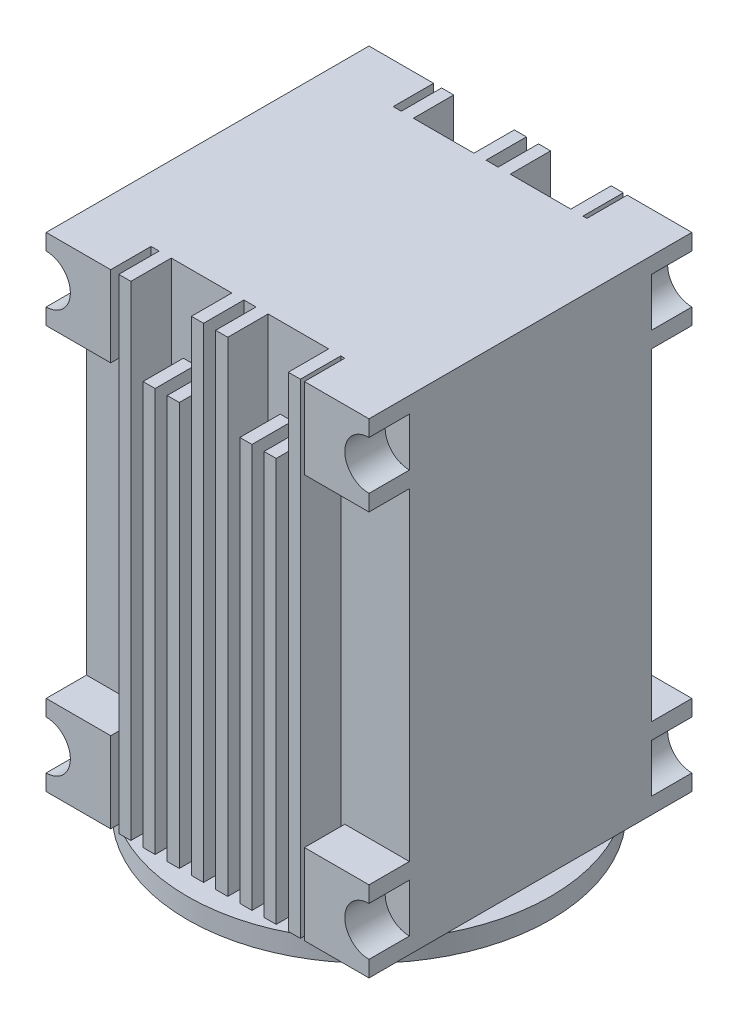
from build123d import *

# Parameters (mm, degrees)
SKETCH1_W           = 40
SKETCH1_H           = 40
BOSS_EXTRUDE1_DEPTH = 30
CUT_EXTRUDE1_DEPTH  = 5
SKETCH3_W           = 1.5
SKETCH3_H           = 5
BOSS_EXTRUDE2_DEPTH = 60
SKETCH4_W           = 4.5
SKETCH4_H           = 10
CUT_EXTRUDE2_DEPTH  = 5
SKETCH5_R           = 3
CUT_EXTRUDE3_DEPTH  = 5
SKETCH6_R           = 22.5
BOSS_EXTRUDE3_DEPTH = 2.5
SKETCH7_R           = 5
CUT_EXTRUDE4_DEPTH  = 15
SKETCH8_R           = 2.5
CUT_EXTRUDE6_DEPTH  = 15
SKETCH9_R           = 1
CUT_EXTRUDE7_DEPTH  = 1.8


with BuildPart() as part:
    # Sketch1 → Boss-Extrude1 (new, symmetric)
    with BuildSketch(Plane(origin=(0, 0, 0), x_dir=(1, 0, 0), z_dir=(0, 1, 0))):
        Rectangle(SKETCH1_W, SKETCH1_H)
    extrude(amount=BOSS_EXTRUDE1_DEPTH, both=True)

    # Sketch2 → Cut-Extrude1 (cut)
    with BuildSketch(Plane(origin=(0, 0, -20), x_dir=(-1, 0, 0), z_dir=(0, 0, -1))):
        Polygon((-12, 30), (12, 30), (12, 20), (20, 20), (20, -20), (12, -20), (12, -30), (-12, -30), (-12, -20), (-20, -20), (-20, 20), (-12, 20), align=None)
    cut_extrude1 = extrude(amount=-CUT_EXTRUDE1_DEPTH, mode=Mode.SUBTRACT)

    # Mirror1: Cut-Extrude1 across plane
    add(cut_extrude1.mirror(Plane.XY), mode=Mode.SUBTRACT)

    # Sketch3 → Boss-Extrude2 (add)
    with BuildSketch(Plane(origin=(0, 30, 0), x_dir=(1, 0, 0), z_dir=(0, 1, 0))):
        with Locations((-10.25, 17.5)):
            Rectangle(SKETCH3_W, SKETCH3_H)
        with Locations((-7.25, 17.5)):
            Rectangle(SKETCH3_W, SKETCH3_H)
        with Locations((-4.25, 17.5)):
            Rectangle(SKETCH3_W, SKETCH3_H)
        with Locations((-1.25, 17.5)):
            Rectangle(SKETCH3_W, SKETCH3_H)
        with Locations((1.75, 17.5)):
            Rectangle(SKETCH3_W, SKETCH3_H)
        with Locations((4.75, 17.5)):
            Rectangle(SKETCH3_W, SKETCH3_H)
        with Locations((7.75, 17.5)):
            Rectangle(SKETCH3_W, SKETCH3_H)
        with Locations((10.75, 17.5)):
            Rectangle(SKETCH3_W, SKETCH3_H)
    boss_extrude2 = extrude(amount=-BOSS_EXTRUDE2_DEPTH)

    # Sketch4 → Cut-Extrude2 (cut)
    with BuildSketch(Plane(origin=(0, 0, -20), x_dir=(-1, 0, 0), z_dir=(0, 0, -1))):
        with Locations((-6.25, 25)):
            Rectangle(SKETCH4_W, SKETCH4_H)
        with Locations((5.75, 25)):
            Rectangle(SKETCH4_W, SKETCH4_H)
    cut_extrude2 = extrude(amount=-CUT_EXTRUDE2_DEPTH, mode=Mode.SUBTRACT)

    # Mirror2: Boss-Extrude2, Cut-Extrude2 across plane
    add(boss_extrude2.mirror(Plane.XY))
    add(cut_extrude2.mirror(Plane.XY), mode=Mode.SUBTRACT)

    # Sketch5 → Cut-Extrude3 (cut)
    with BuildSketch(Plane(origin=(0, 0, -20), x_dir=(-1, 0, 0), z_dir=(0, 0, -1))):
        with Locations((-20, 25)):
            Circle(SKETCH5_R)
        with Locations((20, 25)):
            Circle(SKETCH5_R)
        with Locations((-20, -25)):
            Circle(SKETCH5_R)
        with Locations((20, -25)):
            Circle(SKETCH5_R)
    cut_extrude3 = extrude(amount=-CUT_EXTRUDE3_DEPTH, mode=Mode.SUBTRACT)

    # Mirror3: Cut-Extrude3 across plane
    add(cut_extrude3.mirror(Plane.XY), mode=Mode.SUBTRACT)

    # Sketch6 → Boss-Extrude3 (add)
    with BuildSketch(Plane.XZ.offset(30)):
        with Locations(Location((0, 0, 0), (0, 0, 62.733955549))):
            Circle(SKETCH6_R)
    extrude(amount=BOSS_EXTRUDE3_DEPTH)

    # Sketch7 → Cut-Extrude4 (cut)
    with BuildSketch(Plane.XZ.offset(32.5)):
        with Locations(Location((0, 0, 0), (0, 0, 270))):
            Circle(SKETCH7_R)
    extrude(amount=-CUT_EXTRUDE4_DEPTH, mode=Mode.SUBTRACT)

    # Sketch8 → Cut-Extrude6 (cut)
    with BuildSketch(Plane.ZY.offset(20)):
        with Locations((4.37, 17.51)):
            Circle(SKETCH8_R)
    extrude(amount=-CUT_EXTRUDE6_DEPTH, mode=Mode.SUBTRACT)

    # Sketch9 → Cut-Extrude7 (cut)
    with BuildSketch(Plane.XZ.offset(30)):
        with Locations(Location((-17.5, 17.5, 0), (0, 0, 270))):
            Circle(SKETCH9_R)
        with Locations(Location((-17.5, -17.5, 0), (0, 0, 270))):
            Circle(SKETCH9_R)
        with Locations(Location((17.5, -17.5, 0), (0, 0, 270))):
            Circle(SKETCH9_R)
        with Locations(Location((17.5, 17.5, 0), (0, 0, 270))):
            Circle(SKETCH9_R)
    extrude(amount=-CUT_EXTRUDE7_DEPTH, mode=Mode.SUBTRACT)


solid = part.part
